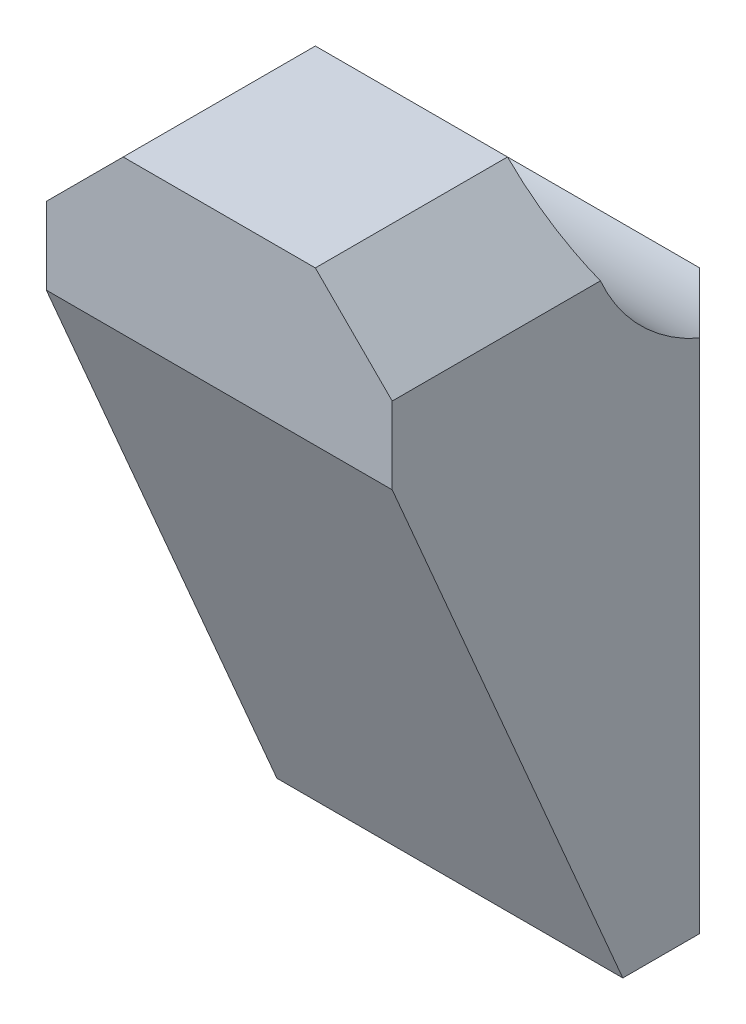
SolidWorks part; units mm, degrees
material "Q235-A"
ref_plane "Front Plane" through (0, 0, 0) normal (0, 0, 1) x (1, 0, 0)
ref_plane "Top Plane" through (0, 0, 0) normal (0, 1, 0) x (1, 0, 0)
ref_plane "Right Plane" through (0, 0, 0) normal (1, 0, 0) x (0, 0, -1)
sketch "Sketch1" plane through (0, 0, 0) normal (1, 0, 0) x (0, 0, -1)
  line L0 (0, 0) -> (0, 65)
  line L1 (-25, 90) -> (-50, 90)
  line L2 (-50, 90) -> (-50, 70)
  line L3 (-50, 70) -> (-20, 0)
  line L4 (-20, 0) -> (0, 0)
  arc A0 (-25, 90) -> (0, 65) centre (0, 90) ccw
  dimension "D1" = 50
  dimension "D2" = 90
  dimension "D3" = 20
  dimension "D4" = 20
  dimension "D5" = 50
extrude "Boss-Extrude1" add sketch "Sketch1" along normal mid plane 45
chamfer "Chamfer1" distance 10 angle 45 4 edges at (-22.5, 32.5, 0) (22.5, 32.5, 0) (22.5, 90, 37.5) (-22.5, 90, 37.5)
